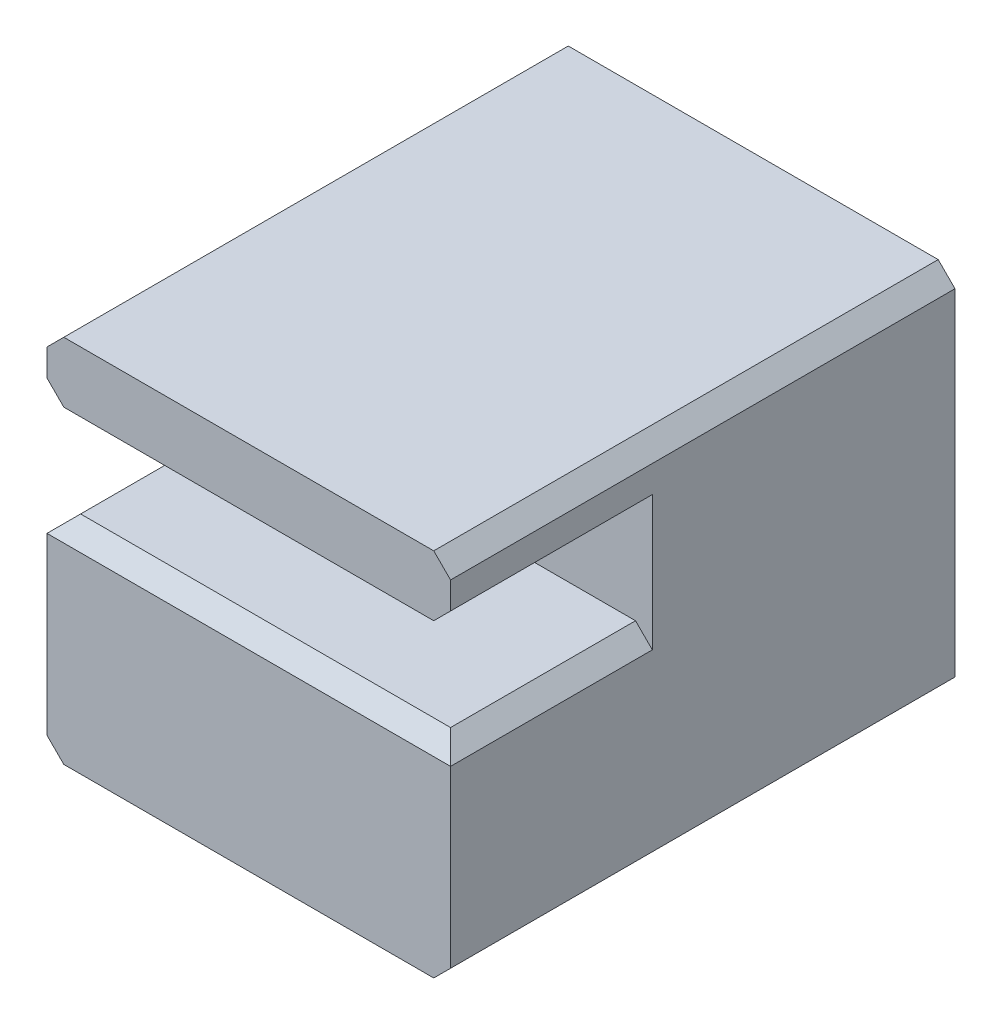
from build123d import *

# Parameters (mm, degrees)
SKETCH_1_R           = 8
EXTRUDE_1_DEPTH      = 7.5
SKETCH_3_R           = 2.5
CUT_EXTRUDE_2_DEPTH  = 12.5
SKETCH_4_OUTSIDE_W   = 23.43
SKETCH_4_OUTSIDE_H   = 23.43
SKETCH_4_OUTSIDE_W_2 = 12
SKETCH_4_OUTSIDE_H_2 = 20.092263618
CUT_EXTRUDE_3_DEPTH  = 19.788294228
SKETCH_5_W           = 16.185662541
SKETCH_5_H           = 6.325725708
CUT_EXTRUDE_4_DEPTH  = 19.027756377
SKETCH_8_W           = 12
SKETCH_8_H           = 2.708497378
EXTRUDE_2_DEPTH      = 15
CHAMFER_1_SIZE       = 0.5
SKETCH_2_W           = 17
SKETCH_2_H           = 3
CUT_EXTRUDE_5_DEPTH  = 6
CHAMFER_2_SIZE       = 0.5


with BuildPart() as part:
    # 草图1 → 凸台-拉伸1 (new, symmetric)
    with BuildSketch(Plane.XY):
        Circle(SKETCH_1_R)
    extrude(amount=EXTRUDE_1_DEPTH, both=True)

    # 草图3 → 切除-拉伸2 (cut)
    with BuildSketch(Plane(origin=(0, 0, -7.5), x_dir=(-1, 0, 0), z_dir=(0, 0, -1))):
        Circle(SKETCH_3_R)
    extrude(amount=-CUT_EXTRUDE_2_DEPTH, mode=Mode.SUBTRACT)

    # 草图4 outside → 切除-拉伸3 (cut, through all)
    with BuildSketch(Plane.XY.offset(7.5)):
        Rectangle(SKETCH_4_OUTSIDE_W, SKETCH_4_OUTSIDE_H)
        Rectangle(SKETCH_4_OUTSIDE_W_2, SKETCH_4_OUTSIDE_H_2, mode=Mode.SUBTRACT)
    extrude(amount=-CUT_EXTRUDE_3_DEPTH, mode=Mode.SUBTRACT)

    # 草图5 → 切除-拉伸4 (cut, through all)
    with BuildSketch(Plane.XY.offset(7.5)):
        with Locations((0.239490277, -6.162862854)):
            Rectangle(SKETCH_5_W, SKETCH_5_H)
    extrude(amount=-CUT_EXTRUDE_4_DEPTH, mode=Mode.SUBTRACT)

    # 草图8 → 凸台-拉伸2 (add)
    with BuildSketch(Plane(origin=(0, 0, -7.5), x_dir=(-1, 0, 0), z_dir=(0, 0, -1))):
        with Locations((0, 6.645751311)):
            Rectangle(SKETCH_8_W, SKETCH_8_H)
    extrude(amount=-EXTRUDE_2_DEPTH)

    # 倒角1
    chamfer_1_edges = [part.edges().sort_by_distance(p)[0] for p in [
        (6, -3, 0),
        (-6, -3, 0),
        (6, 8, 0),
        (-6, 8, 0),
    ]]
    chamfer(chamfer_1_edges, length=CHAMFER_1_SIZE)

    # 草图2 → 切除-拉伸5 (cut)
    with BuildSketch(Plane.XY.offset(7.5)):
        with Locations((0.206171625, 4.7)):
            Rectangle(SKETCH_2_W, SKETCH_2_H)
    extrude(amount=-CUT_EXTRUDE_5_DEPTH, mode=Mode.SUBTRACT)

    # 倒角2
    chamfer_2_edges = [part.edges().sort_by_distance(p)[0] for p in [
        (6, 3.2, 4.5),
        (6, 6.2, 4.5),
        (-6, 6.2, 4.5),
        (-6, 3.2, 4.5),
        (0, 3.2, 7.5),
    ]]
    chamfer(chamfer_2_edges, length=CHAMFER_2_SIZE)


solid = part.part
